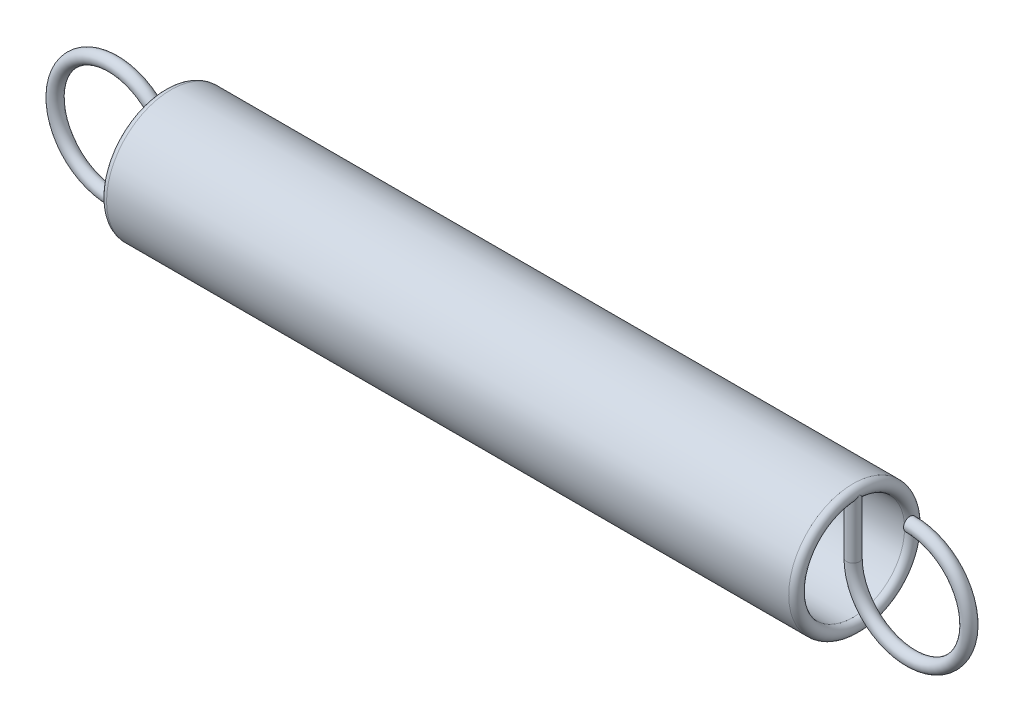
from build123d import *

# Parameters (mm, degrees)
SKETCH2_W      = 0.25
SKETCH2_H      = 2.25
SKETCH3_R      = 0.25
REVOLVE3_ANGLE = 271
SKETCH4_W      = 0.25
SKETCH4_H      = 2.25
SKETCH5_R      = 0.25
REVOLVE5_ANGLE = 271


with BuildPart() as part:
    # Sketch1 → Revolve1 (revolve)
    with BuildSketch(Plane.XY, mode=Mode.PRIVATE) as revolve1_sk:
        with BuildLine():
            Line((4.25, 2), (30.75, 2))
            ThreePointArc((30.75, 2), (31, 2.25), (30.75, 2.5))
            Line((30.75, 2.5), (4.25, 2.5))
            ThreePointArc((4.25, 2.5), (4, 2.25), (4.25, 2))
        make_face()
    revolve(revolve1_sk.sketch.rotate(Axis((31, 0, 0), (-1, 0, 0)), 270), axis=Axis((31, 0, 0), (-1, 0, 0)))

    # Sketch2 → Revolve2 (revolve)
    with BuildSketch(Plane.XY, mode=Mode.PRIVATE) as revolve2_sk:
        with Locations((30.875, 1.125)):
            Rectangle(SKETCH2_W, SKETCH2_H)
    revolve(revolve2_sk.sketch.rotate(Axis((30.75, 0, 0), (0, 1, 0)), 270), axis=Axis((30.75, 0, 0), (0, 1, 0)))

    # Sketch3 → Revolve3 (revolve)
    with BuildSketch(Plane(origin=(0, 0, 0), x_dir=(1, 0, 0), z_dir=(0, 1, 0))):
        with Locations(Location((30.75, 0, 0), (0, 0, 269.999999944))):
            Circle(SKETCH3_R)
    revolve(axis=Axis((33, 0, -2.5), (0, 0, 1)), revolution_arc=REVOLVE3_ANGLE)

    # Sketch4 → Revolve4 (revolve)
    with BuildSketch(Plane.XY, mode=Mode.PRIVATE) as revolve4_sk:
        with Locations((4.375, -1.125)):
            Rectangle(SKETCH4_W, SKETCH4_H)
    revolve(revolve4_sk.sketch.rotate(Axis((4.25, -2.25, 0), (0, 1, 0)), 90), axis=Axis((4.25, -2.25, 0), (0, 1, 0)))

    # Sketch5 → Revolve5 (revolve)
    with BuildSketch(Plane(origin=(0, 0, 0), x_dir=(1, 0, 0), z_dir=(0, 1, 0))):
        with Locations(Location((4.25, 0, 0), (0, 0, 90))):
            Circle(SKETCH5_R)
    revolve(axis=Axis((2, 0, 2.5), (0, 0, 1)), revolution_arc=REVOLVE5_ANGLE)


solid = part.part
